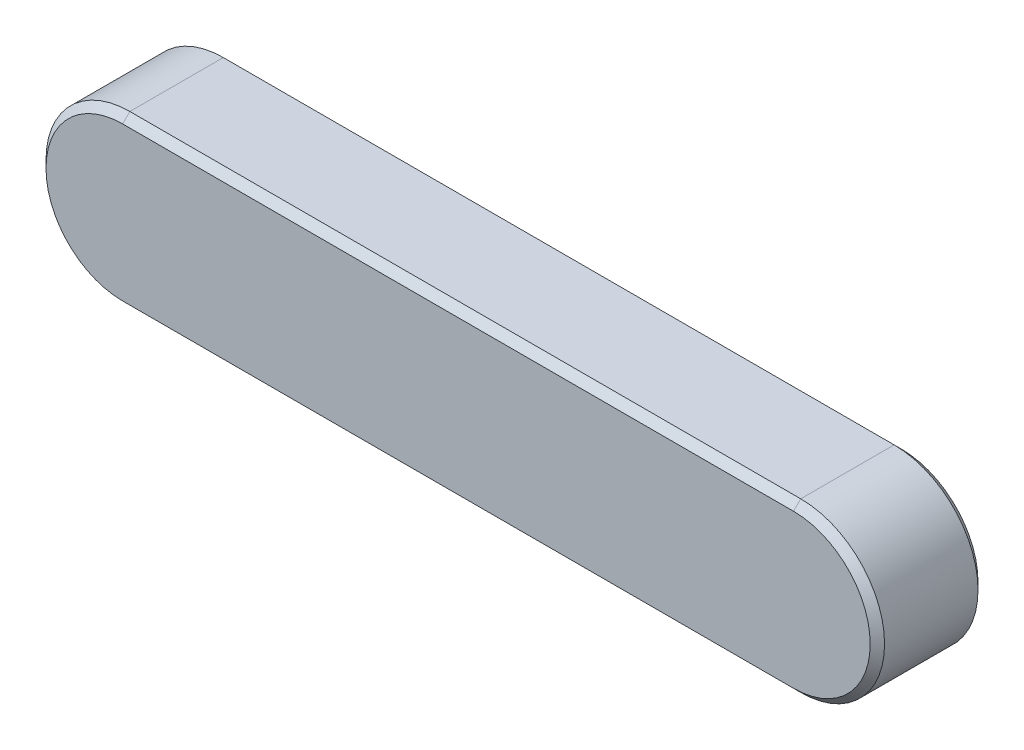
SolidWorks part; units mm, degrees
ref_plane "Front" through (0, 0, 0) normal (0, 0, 1) x (1, 0, 0)
ref_plane "Top" through (0, 0, 0) normal (0, 1, 0) x (1, 0, 0)
ref_plane "Right" through (0, 0, 0) normal (1, 0, 0) x (0, 0, -1)
sketch "Sketch1" plane through (0, 0, 0) normal (0, 0, 1) x (1, 0, 0)
  line L0 (-56, 7) -> (0, 7)
  line L1 (0, -7) -> (-56, -7)
  arc A0 (0, 7) -> (0, -7) centre (0, 0) cw
  arc A1 (-56, -7) -> (-56, 7) centre (-56, 0) cw
  dimension "L" = 70
  dimension "b" = 14
extrude "BaseKey" add sketch "Sketch1" along normal mid plane 9
sketch "Sketch2" plane through (0, 0, 0) normal (0, 0, 1) x (1, 0, 0)
  line L1 (-63, 7) -> (7, 7)
  line L2 (-63, 7) -> (-63, -7)
  line L3 (-63, -7) -> (7, -7)
  line L4 (7, 7) -> (7, -7)
  line L6 (0, -7) -> (-56, -7) construction
  line L7 (-56, 7) -> (0, 7) construction
  arc A2 (0, -7) -> (0, 7) centre (0, 0) ccw construction
  arc A3 (-56, 7) -> (-56, -7) centre (-56, 0) ccw construction
extrude "Extrude1" [suppressed] add sketch "Sketch2" along normal mid plane 9
sketch "Sketch3" plane through (0, 0, 0) normal (0, 0, 1) x (1, 0, 0)
  line L0 (7, 7) -> (-56, 7)
  line L1 (-56, -7) -> (7, -7)
  line L2 (7, -7) -> (7, 7)
  line L5 (-56, 7) -> (0, 7) construction
  arc A0 (-56, 7) -> (-56, -7) centre (-56, 0) ccw
  arc A1 (0, -7) -> (0, 7) centre (0, 0) ccw construction
  arc A4 (-56, 7) -> (-56, -7) centre (-56, 0) ccw construction
extrude "Extrude2" [suppressed] add sketch "Sketch3" along normal mid plane 9
chamfer "Chamfer1" distance 0.6 angle 45 8 edges at (7, 0, -4.5) (-28, -7, -4.5) (-63, 0, -4.5) (-28, 7, -4.5) (-63, 0, 4.5) (-28, -7, 4.5) (7, 0, 4.5) (-28, 7, 4.5)
equation "\"D1@Extrude1\"=\"h@BaseKey\""
equation "\"D1@Extrude2\"=\"h@BaseKey\""
